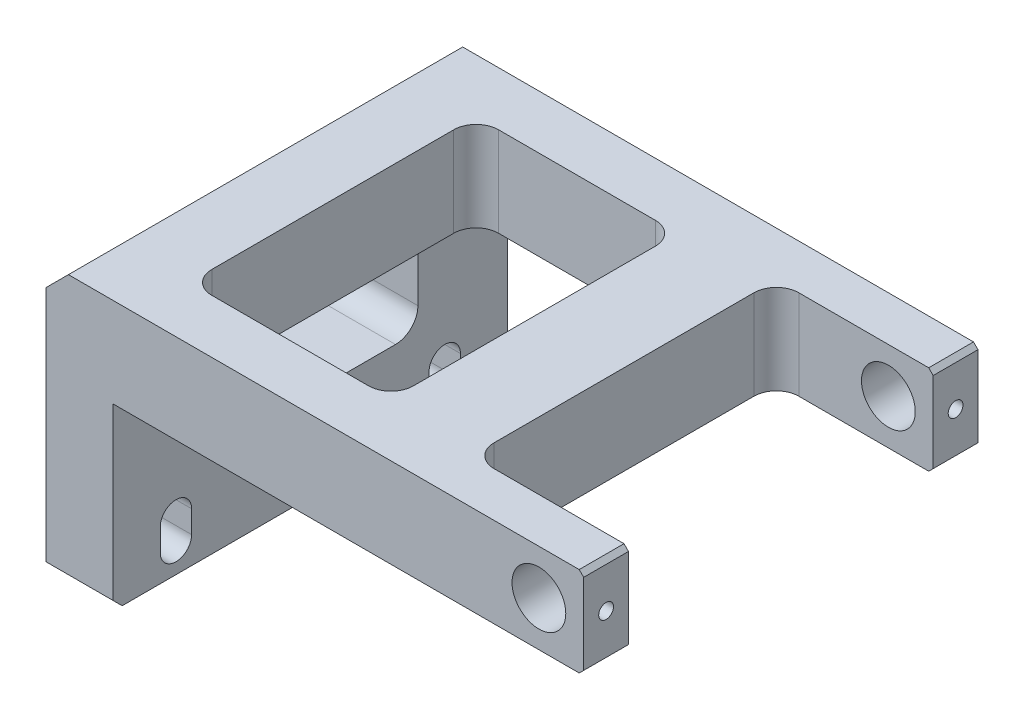
from build123d import *

# Parameters (mm, degrees)
SKETCH1_R             = 6
BOSS_EXTRUDE1_DEPTH   = 44
SKETCH2_W             = 70
SKETCH2_H             = 68
CUT_EXTRUDE1_DEPTH    = 142.194900758
CUT_EXTRUDE2_DEPTH    = 142.194900758
M4_TAPPED_HOLE1_D     = 3.3
M4_TAPPED_HOLE1_DEPTH = 10.1
M4_TAPPED_HOLE1_TIP   = 0.991420021
SKETCH7_W             = 45
SKETCH7_H             = 64
CUT_EXTRUDE4_DEPTH    = 142.194900874
SKETCH8_W             = 48
SKETCH8_H             = 20
CUT_EXTRUDE5_DEPTH    = 142.194900874
CHAMFER1_SIZE         = 5
CHAMFER2_SIZE         = 2
CHAMFER3_SIZE         = 1
FILLET1_R             = 5


with BuildPart() as part:
    # Sketch1 → Boss-Extrude1 (new, symmetric)
    with BuildSketch(Plane.XY):
        Polygon((0, 0), (0, 60), (120, 60), (120, 40), (15, 40), (15, 0), align=None)
        with Locations((110, 50)):
            Circle(SKETCH1_R, mode=Mode.SUBTRACT)
    extrude(amount=BOSS_EXTRUDE1_DEPTH, both=True)

    # Sketch2 → Cut-Extrude1 (cut, through all)
    with BuildSketch(Plane(origin=(0, 60, 0), x_dir=(1, 0, 0), z_dir=(0, 1, 0))):
        with Locations((120, 0)):
            Rectangle(SKETCH2_W, SKETCH2_H)
    extrude(amount=-CUT_EXTRUDE1_DEPTH, mode=Mode.SUBTRACT)

    # Sketch3 → Cut-Extrude2 (cut, through all)
    with BuildSketch(Plane.ZY):
        with BuildLine():
            Line((-33.5, 6), (-33.5, 11))
            ThreePointArc((-33.5, 11), (-30, 14.5), (-26.5, 11))
            Line((-26.5, 11), (-26.5, 6))
            ThreePointArc((-26.5, 6), (-30, 2.5), (-33.5, 6))
        make_face()
        with BuildLine():
            Line((33.5, 6), (33.5, 11))
            ThreePointArc((33.5, 11), (30, 14.5), (26.5, 11))
            Line((26.5, 11), (26.5, 6))
            ThreePointArc((26.5, 6), (30, 2.5), (33.5, 6))
        make_face()
    extrude(amount=-CUT_EXTRUDE2_DEPTH, mode=Mode.SUBTRACT)

    # M4 Tapped Hole1
    with Locations(Plane(origin=(120, 0, 0), x_dir=(0, 0, -1), z_dir=(1, 0, 0))):
        with Locations((-39, 50), (39, 50)):
            Hole(M4_TAPPED_HOLE1_D / 2, depth=M4_TAPPED_HOLE1_DEPTH)
            with Locations((0, 0, -(M4_TAPPED_HOLE1_DEPTH + M4_TAPPED_HOLE1_TIP / 2))):  # 118° drill point
                Cone(0, M4_TAPPED_HOLE1_D / 2, M4_TAPPED_HOLE1_TIP, mode=Mode.SUBTRACT)

    # Sketch7 → Cut-Extrude4 (cut, through all)
    with BuildSketch(Plane(origin=(0, 60, 0), x_dir=(-1, 0, 0), z_dir=(0, 1, 0))):
        with Locations((-42.5, 0)):
            Rectangle(SKETCH7_W, SKETCH7_H)
    extrude(amount=-CUT_EXTRUDE4_DEPTH, mode=Mode.SUBTRACT)

    # Sketch8 → Cut-Extrude5 (cut, through all)
    with BuildSketch(Plane.ZY):
        with Locations((0, 30)):
            Rectangle(SKETCH8_W, SKETCH8_H)
    extrude(amount=-CUT_EXTRUDE5_DEPTH, mode=Mode.SUBTRACT)

    # Chamfer1
    chamfer1_edges = [part.edges().sort_by_distance(p)[0] for p in [
        (0, 60, 0),
    ]]
    chamfer(chamfer1_edges, length=CHAMFER1_SIZE)

    # Chamfer2
    chamfer2_edges = [part.edges().sort_by_distance(p)[0] for p in [
        (7.5, 0, 44),
        (7.5, 0, -44),
    ]]
    chamfer(chamfer2_edges, length=CHAMFER2_SIZE)

    # Chamfer3
    chamfer3_edges = [part.edges().sort_by_distance(p)[0] for p in [
        (120, 60, 39),
        (120, 40, 39),
        (120, 60, -39),
        (120, 40, -39),
    ]]
    chamfer(chamfer3_edges, length=CHAMFER3_SIZE)

    # Fillet1
    fillet1_edges = [part.edges().sort_by_distance(p)[0] for p in [
        (7.5, 40, 24),
        (7.5, 20, 24),
        (7.5, 20, -24),
        (7.5, 40, -24),
        (85, 50, 34),
        (85, 50, -34),
        (65, 50, -32),
        (65, 50, 32),
        (20, 50, 32),
        (20, 50, -32),
    ]]
    fillet(fillet1_edges, radius=FILLET1_R)


solid = part.part
